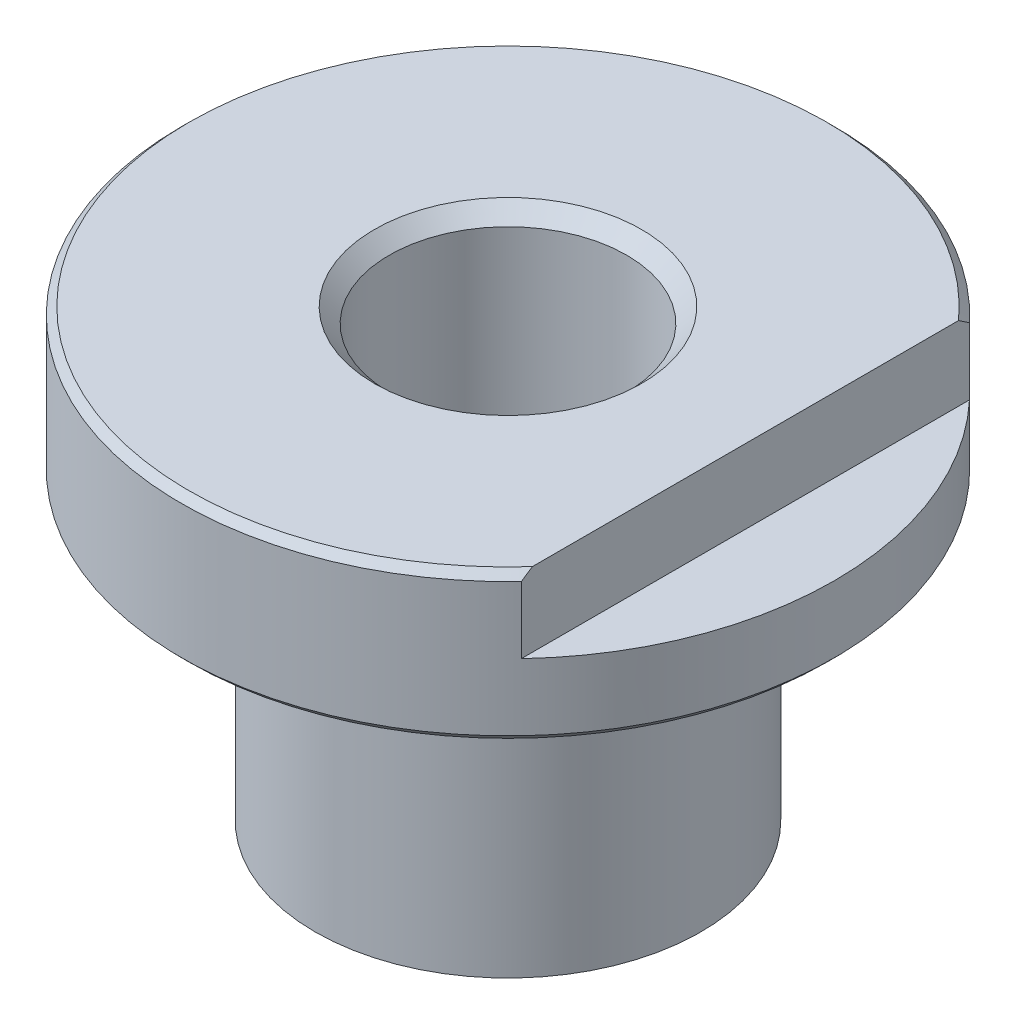
from build123d import *

# Parameters (mm, degrees)
CHAMFER1_SIZE      = 0.5
CHAMFER2_SIZE      = 1
SKETCH2_W          = 20.223718868
SKETCH2_H          = 51.853895089
CUT_EXTRUDE1_DEPTH = 5


with BuildPart() as part:
    # Sketch1 → Revolve1 (revolve)
    with BuildSketch(Plane.XY, mode=Mode.PRIVATE) as revolve1_sk:
        Polygon((-22, 18.531875125), (-22, 8.531875125), (-13, 8.531875125), (-13, -11.468124875), (-8, -11.468124875), (-8, 18.531875125), align=None)
    revolve(revolve1_sk.sketch.rotate(Axis((0, 40.811378681, 0), (0, -1, 0)), 270), axis=Axis((0, 40.811378681, 0), (0, -1, 0)))

    # Chamfer1
    chamfer1_edges = [part.edges().sort_by_distance(p)[0] for p in [
        (0, 8.531875125, -22),
        (0, 18.531875125, -22),
    ]]
    chamfer(chamfer1_edges, length=CHAMFER1_SIZE)

    # Chamfer2
    chamfer2_edges = [part.edges().sort_by_distance(p)[0] for p in [
        (0, 18.531875125, -8),
    ]]
    chamfer(chamfer2_edges, length=CHAMFER2_SIZE)

    # Sketch2 → Cut-Extrude1 (cut)
    with BuildSketch(Plane(origin=(0, 18.531875125, 0), x_dir=(1, 0, 0), z_dir=(0, 1, 0))):
        with Locations((26.111859434, -0.909717457)):
            Rectangle(SKETCH2_W, SKETCH2_H)
    extrude(amount=-CUT_EXTRUDE1_DEPTH, mode=Mode.SUBTRACT)


solid = part.part
